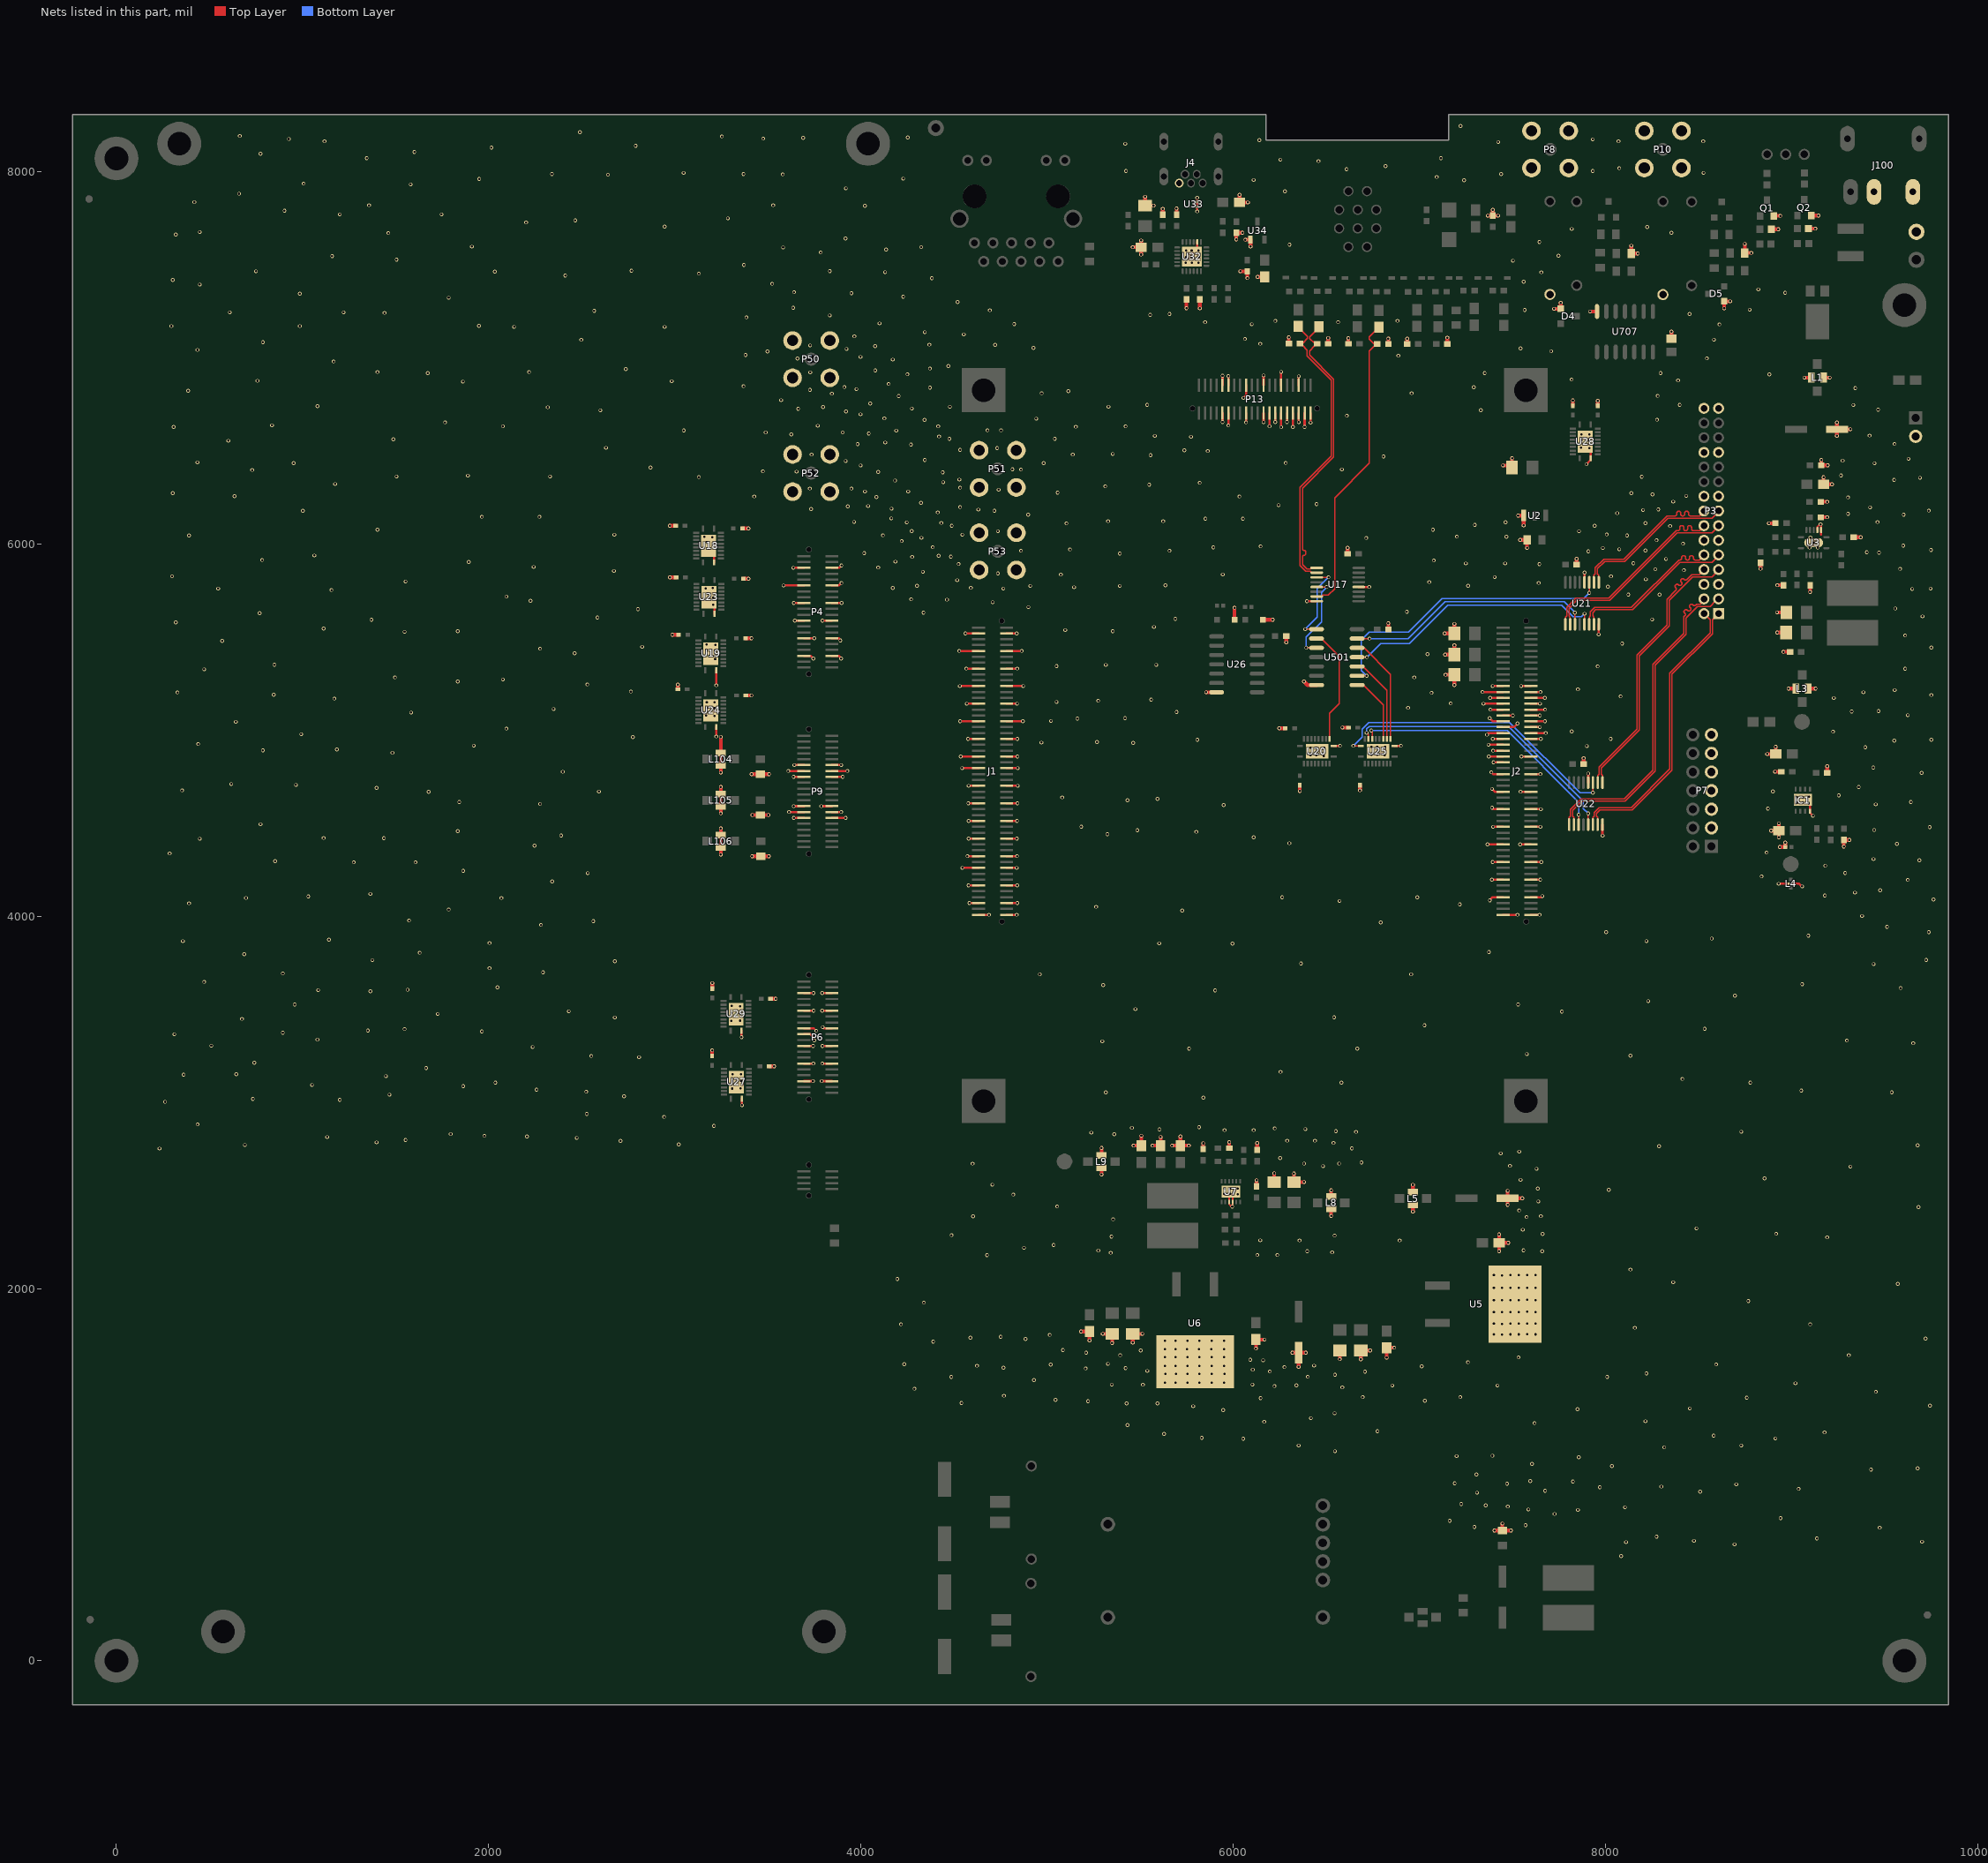
[diagram p0: the nets of this part, all layers, seen from the top]
# Altium PCB MISC82191.PcbDoc (part 6 of 9)
Units mil, origin at the board's own origin, x right, y up, seen from the top; angles counter-clockwise.
Board outline 10078.74 x 8543.31 mil, 4 copper layers (Top Layer, GND, POWER, Bottom Layer); 238 components, 299 nets, 1297 pads, 1665 vias.

## Via types
v1: diameter 20, hole 12, Top Layer to Bottom Layer, 1664 vias
v2: diameter 40, hole 20, Top Layer to Bottom Layer, 1 vias

## Nets (pads, with @x,y where several pads share a name; then routed paths per layer and width w, separated by ;. In a path a pad name is that pad's centre, name@x,y a point inside that pad or via, vN(x,y) a via of type N, cw(c..) or ccw(c..) an arc to the next point about the centre after c; other vN are vias at no path point) (continued)
DGND: (continued)
  other v1: 8084,563 8694,626 8110,638 9701,640 8475,645 9136,657 8275,667 9473,715 7296,719 7571,729 7163,752 8941,767 7726,789 7852,811 7586,813 8105,825 7475,829 7357,835 7225,842 7310,903 8509,909 7676,913 9038,924 7970,932 8300,936 8703,948 7471,951 7190,954 7825,963 7596,966 7307,1001 9427,1027 9677,1034 8035,1046 7605,1058 7857,1094 7200,1100 7393,1102 6547,1126 8316,1147 6352,1157 8730,1157 6054,1193 8913,1195 5831,1198 8581,1210 5629,1219 9177,1227 6775,1234 5432,1267 7619,1277 6167,1284 8215,1287 6417,1304 6544.78,1329.78 5946,1347 7850,1352 8453,1356 5785,1368 9744,1371 5427,1383 5593,1383 4540,1385 5220,1395 7030,1397 5045,1402 6146.78,1411.78 8759,1414 6696,1417 7220,1417 4768,1424 9453,1445 4288,1462 6586,1469 6221.78,1476.16 6855,1479 7420,1479 6339.78,1480.16 5514.78,1483.16 5347.78,1484.16 6103.78,1484.16 9021,1491 5633.78,1495.16 5690.78,1495.16 5753.78,1495.16 5817.78,1495.16 5883.78,1495.16 5951.78,1495.16 4929,1508 4485,1525 8009,1525 6400.78,1526.16 6547,1537 5634.78,1541.16 5691.78,1541.16 5754.78,1541.16 5818.78,1541.16 5884.78,1541.16 5952.78,1541.16 8220,1544 6196.78,1554.16 6708,1554 5538.78,1557.16 6104.78,1564.16 5207.78,1571.16 5421.78,1572.16 4766,1575 6274.78,1578.16 7013,1582 5633.78,1584.16 5690.78,1584.16 5753.78,1584.16 5817.78,1584.16 5883.78,1584.16 5951.78,1584.16 4624,1585 6434.78,1586.16 5019.78,1591.16 8595,1592 4232,1594 5326.78,1595.16 7261,1604 6160.78,1614.16 6091.78,1617.16 7533,1630 5633.78,1631.16 5690.78,1631.16 5753.78,1631.16 5817.78,1631.16 5883.78,1631.16 5951.78,1631.16 5392.78,1642.16 9307,1642 5209.78,1655.16 5502.78,1667.16 5084.78,1670.16 5632.78,1674.16 5689.78,1674.16 5752.78,1674.16 5816.78,1674.16 5882.78,1674.16 5950.78,1674.16 4388,1715 5633.78,1719.16 5690.78,1719.16 5753.78,1719.16 5817.78,1719.16 5883.78,1719.16 5951.78,1719.16 4884,1729 9720,1731 4588,1736 4751,1741 5013.78,1751.16 7445.4,1752.78 7400.4,1753.78 7488.4,1753.78 7535.4,1753.78 7624.4,1753.78 7578.4,1754.78 8158,1789 4215,1808 9100,1808 7445.4,1809.78 7400.4,1810.78 7488.4,1810.78 7535.4,1810.78 7624.4,1810.78 7578.4,1811.78 7445.4,1872.78 7400.4,1873.78 7488.4,1873.78 7535.4,1873.78 7624.4,1873.78 7578.4,1874.78 4338,1924 8768,1933 7445.4,1936.78 7400.4,1937.78 7488.4,1937.78 7535.4,1937.78 7624.4,1937.78 7578.4,1938.78 7445.4,2002.78 7400.4,2003.78 7488.4,2003.78 7535.4,2003.78 7624.4,2003.78 7578.4,2004.78 9571,2025 8364,2034 4195.53,2051 7445.4,2070.78 7400.4,2071.78 7488.4,2071.78 7535.4,2071.78 7624.4,2071.78 7578.4,2072.78 8134,2102 4677,2179 6129.78,2180.16 6236.78,2180.16 5341.78,2192.16 6531.78,2194.16 6397.78,2200.16 7659.78,2200.78 5275.78,2204.16 7559.4,2205.78 4876,2219 5035,2234 6356.78,2258.16 6894.78,2258.41 6145.78,2259.16 9191,2275 5345.78,2279.16 6544.78,2284.16 4487,2287 7662.78,2292.78 8917,2294 7555.4,2315.78 8489,2323 5354.78,2372.16 7576.4,2383.78 4602,2388 7652.78,2388.78 7535.78,2419.78 9682,2438 5054,2441 7639.78,2467.78 4819,2505 6023.78,2506.16 5951.78,2509.16 5984.78,2509.16 8018,2530 5984.78,2536.16 7636.78,2536.78 5952.78,2538.16 6023.78,2538.16 4706,2558 7543.78,2583.78 8855,2592 7629.78,2642.78 9316,2655 6482.78,2657.16 7487.4,2658.78 4600,2671 6380.78,2671.16 6568.78,2671.16 6688.78,2677.16 6251.78,2701.16 7437.4,2725.78 7536.4,2735.78 231,2752 6637.78,2753.16 8288,2765 9677,2770 690,2771 3021,2774 6538.78,2782.16 1397,2785 2708,2793 6289.78,2794.16 6439.78,2794.16 1553,2798 2473,2809 1132,2814 2206,2817 1977,2820 5360.78,2829.16 1796,2830 5237.78,2837.16 6659.78,2841.16 8730,2842 6551.78,2845.16 5953.78,2851.16 6109.78,2851.16 5603.78,2855.16 6387.78,2856.16 6222.78,2860.16 5455.78,2863.16 5816.78,2867.16 3210,2874 436,2882 2942,2922 2527,2938 261,3003 1199.78,3014.16 732.78,3018.16 5840,3025 2727,3033 1467,3041 5316,3054 9538,3054 2524,3057 9052,3063 2257,3068 3308.78,3074.16 3352.78,3075.16 1863,3087 1050.78,3093.16 2036,3106 6581,3106 8778,3106 3308.78,3115.16 3354.78,3115.16 8413,3126 1448,3141 361,3149 3309.78,3150.16 3354.78,3150.16 644,3151 6254,3164 1664,3184 740.78,3213.16 2808,3243 2551,3249 8134,3251 7577.78,3259.16 5763,3289 6667,3289 2236,3297 509.78,3304.16 9653,3318 5297,3328 9297,3332 1079.78,3337.16 310.78,3366.16 893.78,3374.16 1963,3381 1351,3386 1548,3394 8533,3395 7028,3414 3303.78,3438.16 3349.78,3439.16 674.78,3448.16 2678,3456 6542,3457 1726,3475 3349.78,3479.16 3305.78,3480.16 7765.78,3488.16 2430,3489 5475,3501 3349.78,3517.16 3304.78,3518.16 957.78,3525.16 7530.78,3526.16 8230,3544 8696,3573 1364,3597 5903,3602 1083.78,3603.16 1564,3605 9586,3614 2047,3618 5302,3630 9057,3635 471.78,3647.16 4961,3688 6956,3688 893.78,3692.16 2292,3699 2004,3721 9441,3743 6364,3746 2678,3758 1375,3764 9723,3765 686.78,3796.16 1629,3804 7374,3808 5995.78,3852.41 5602.78,3854.41 2004,3856 356.78,3866.16 8220,3866 1141.78,3874.16 8571,3880 9090,3895 8004,3914 9737,3914 9513,3943 2281,3953 6792,3967 2562,3974 1572,3977 9379,4001 5725.78,4030.16 1785,4036 5263.78,4050.16 7217.78,4064.16 389.78,4069.16 6571,4082 9763,4090 695.78,4098.16 2068,4098 6263,4102 6989,4102 1030.78,4106.16 9178.78,4111.16 1364,4120 9340.78,4127.16 9475.78,4139.16 2341,4187 9624,4195 8838.78,4214.16 2532,4231 9287.78,4232.16 1863,4244 9180.78,4271.16 1275,4290 1607,4290 852.78,4296.16 9687,4301 9439.78,4307.16 285.78,4337.16 8865.78,4342.16 2246,4379 9566,4388 6302,4392 447.78,4416.16 1437,4419 1112.78,4420.16 6110,4424 2389,4433 5324,4441 5802,4453 1834,4457 5485,4462 9443.78,4463.16 9742,4479 5184,4481 773.78,4494.16 8872.78,4578.16 5949,4597 9451.78,4601.16 2276,4603 9092.78,4607.16 9028.78,4610.16 9061.78,4611.16 1842,4614 9641,4614 5432,4623 5593,4630 5081,4638 9060.78,4638.16 9028.78,4639.16 9093.78,4641.16 9253.78,4649.16 1677,4668 2592,4670 8899.78,4670.16 352.78,4676.16 1397,4689 9360.78,4694.16 964.78,4705.16 616.78,4710.16 9699,4770 2398,4776 9439,4799 6487.78,4861.16 6414.78,4864.16 6446.78,4864.16 6814.78,4865.16 6741.78,4868.16 6773.78,4868.16 1483,4878 786.78,4891.16 1183.78,4896.16 6414.78,4906.16 6446.78,4906.16 6488.78,4906.16 9395.78,4907.16 6741.78,4910.16 6773.78,4910.16 6815.78,4910.16 7900,4914 1920,4916 438.78,4925.16 5463,4931 4970,4933 5268,4936 9552,4943 5807,4948 9751,4948 8028,4953 2775,4962 992.78,4978.16 9222.78,4991.16 7819,4993 2095,5008 641.78,5044.16 5021,5049 5162.78,5061.16 5418.78,5064.16 3213.78,5076.16 3168.78,5077.16 9624,5080 1583,5094 5696,5097 9322.78,5099.16 9466.78,5102.16 2349,5113 3171.78,5118.16 3213.78,5118.16 6939.78,5119.16 7168.78,5143.16 3171.78,5150.16 3213.78,5150.16 5050.78,5151.16 5274.78,5157.16 5558.78,5163.16 1170.78,5169.16 9226.78,5172.16 8081,5181 9751,5188 844.78,5189.16 7065.78,5200.16 327.78,5202.16 9386,5203 2764,5207 9554,5215 7852,5219 2530,5245 1834,5261 2076,5272 1496,5283 6972.78,5283.16 471.78,5326.16 9610,5330 7958,5342 5050.78,5344.16 5315.78,5350.16 5586.78,5350.16 848.78,5351.16 3216.78,5381.16 3186.78,5398.16 7043.78,5408.16 2462,5412 3216.78,5426.16 3170.78,5427.16 2276,5437 9751,5443 2824,5447 3217.78,5457.16 3169.78,5459.16 8090,5465 567.78,5479.16 9610,5508 1548,5528 1834,5531 5352.78,5531.16 5097.78,5537.16 1112.78,5545.16 5574,5554 318.78,5578.16 1370,5593 8251,5594 5689,5597 2584,5604 9703,5611 769.78,5628.16 4335.78,5630.41 6933,5635 2802,5650 9557,5653 4899.78,5660.41 3206.78,5674.16 4707.78,5686.41 2225,5695 4462.78,5700.41 4269.78,5702.41 3205.78,5710.16 2095,5717 8123,5728 8291,5728 3177.78,5732.16 1154.78,5752.16 9648,5758 546.78,5760.16 3165.78,5760.16 4764.78,5760.16 9747,5760 3203.78,5763.16 4170.78,5763.16 4590.78,5764.16 5144.78,5767.16 8013,5770 4909.78,5774.16 5390.78,5774.16 4300.78,5775.41 7262,5775 5635.78,5777.16 7641,5790 7053,5795 1553,5798 4516.78,5805.16 8217,5810 7405,5822 298.78,5826.16 8030,5826 5073.78,5835.41 5943.78,5836.16 4735.78,5841.16 4332.78,5850.16 2673,5855 8422,5859 8268,5864 9583,5866 4092.78,5873.16 2241,5876 7645,5891 4524.78,5892.16 7250,5895 7461,5895 8150,5896 1893,5903 4184.78,5904.41 7078,5911 782.78,5913.16 8325,5919 4274.78,5930.16 4482.78,5931.41 4417.78,5936.16 1063.78,5938.16 5390.78,5948.16 4017.78,5950.78 9469.78,5953.16 9403.78,5955.16 7908,5960 4859.78,5963.16 5657.78,5963.16 8215,5965 9749,5967 5122.78,5970.16 8074,5971 3182.78,5975.16 7986,5978 9096.78,5980.16 9140.78,5980.16 5893,5981 4385.78,5982.41 6146.78,5987.16 9600,5991 3206.78,6000.16 8417,6001 9116.78,6007.16 3171.78,6010.16 4218.78,6015.16 8275,6020 4324.78,6032.41 6714.78,6032.16 9100.78,6034.16 3201.78,6035.16 3157.78,6038.16 7468,6038 7202,6039 389.78,6045.16 8116,6045 4117.78,6046.41 2675,6049 4544.78,6049.41 8007,6051 4735.78,6068.16 7858,6068 4272.78,6069.16 1402,6076 7073,6076 8347.78,6096 4487.78,6097.16 7942,6097 7298,6102 5103.78,6110.16 4431.78,6112.41 8215,6112 4245.78,6115.41 7463,6116 9461.78,6117.16 3962.78,6117.78 5327.78,6122.16 5623.78,6122.16 5850.78,6135.16 6052,6135 4162.78,6137.16 1963,6146 2273,6146 4898.78,6157.16 9602,6157 9303.78,6161.16 8063,6165 4412.78,6169.16 1001.78,6178.16 4716.78,6178.16 9737,6179 8202,6182 4630.78,6184.16 8284,6185 3732.78,6188 4164.78,6189.41 9421.78,6196.16 4532.78,6198.16 3928.78,6201.78 4037.78,6203.41 6243.78,6208.16 6447.78,6214.16 4322.78,6220.41 8364,6227 9303.78,6250.16 4082.78,6251.41 3427,6255 6033,6255 633.78,6256.16 8434,6258 8253,6266 302.78,6273.16 8139,6273 5056.78,6275.16 4021.78,6281.41 4253.78,6281.41 4739.78,6291.16 3724.78,6297.41 3948.78,6297.41 4532.78,6302.16 5312.78,6309.16 5548.78,6318.16 1174.78,6322.16 5819.78,6328.16 4441.78,6331.16 4183.78,6340.41 9551,6344 4528.78,6345.41 9690,6355 3129,6359 8195,6361 1505,6362 2330,6362 1888,6367 9265.78,6368.16 4439.78,6384.41 4092.78,6386.41 3653.78,6388.41 3473,6390 728.78,6397.16 4859.78,6399.16 6583.78,6400.16 4813.78,6401.41 2870,6410 3998.78,6421.41 9446,6433 951.78,6434.16 4981.78,6434.41 6281.78,6435.16 434.78,6438.16 3917.78,6445.41 9273.78,6447.16 4342.78,6450.41 9628,6457 6807.78,6470.16 5555.78,6477.16 3734.78,6480.16 5137.78,6480.16 5352.78,6483.16 5863.78,6499.16 5737.78,6502.41 4532.78,6505.16 4731.78,6515.16 7913.78,6515.16 2630,6516 7868.78,6516.16 4268.78,6533.41 3981.78,6535.78 9553,6537 4130.78,6544.41 600.78,6554.16 7871.78,6557.16 7913.78,6557.16 1488,6562 5041.78,6564.41 4474.78,6564.78 5772.78,6575.41 4419.78,6577.41 5578.78,6580.41 9419,6582 3625.78,6588.16 7871.78,6589.16 7913.78,6589.16 4041.78,6593.41 3487.78,6598.78 3901.78,6598.78 4189.78,6608.41 3048,6610 4679.78,6610.41 4752.78,6610.41 306.78,6628.16 5154.78,6629.41 5421.78,6631.41 2076,6632 4414.78,6631.78 3767.78,6634.78 835.78,6637.16 1766,6653 4341.78,6666.41 8277,6667 4941.78,6672.41 4125.78,6674.41 6610.78,6688.41 3997.78,6696.41 3919.78,6711.78 2600,6718 7330.78,6718.16 9465,6721 3662.78,6725.78 4273.78,6727.41 2317,6734 3796.78,6735.41 4477.78,6736.41 5329.78,6736.41 1079.78,6740.16 9332,6746 5537.78,6747.41 8399,6747 4049.78,6754.41 3570.78,6772.41 4202.78,6794.41 8280,6795 3843.78,6807.16 4970.78,6809.41 6958.78,6809.16 5113.78,6820.41 385.78,6823.16 3725.78,6827.78 3975.78,6831.41 9342,6837 4370.78,6839.16 3910.78,6842.4 7292.78,6842.16 3368.78,6847.41 4148.78,6859.41 1861,6872 2983,6874 757.78,6876.16 8390,6878 7817.78,6883.16 8880.78,6910.16 4249.78,6911.16 1672,6918 7351,6918 8296,6918 3727.78,6921.41 1402,6923 2217,6923 4076.78,6931.41 2737,6939 4370.78,6942.16 4469.78,6955.41 1166.78,6980.16 4170.78,6990.16 3658.78,6995.41 8545,6996.81 3997.78,7004.41 6887.78,7011.16 3379.78,7014.41 3497.78,7033.41 7708,7035 434.78,7042.16 3922.78,7047.41 7544,7050 4926.78,7053.16 4075.78,7062.16 3726.78,7066.41 4720.78,7069.16 4367.78,7070.16 6145.78,7075.16 786.78,7083.16 2497,7096 8583,7097 6063,7101 3964.78,7115.16 4552.78,7125.16 4342.78,7137.16 2136,7166 2945,7166 294.78,7170.16 984.78,7170.16 1947,7171 8612,7179 6099.78,7180.16 4823.78,7181.16 4099.78,7184.41 5849,7191 6563.78,7191.16 6227,7198 6882.78,7198.16 3384.78,7217.41 3832.78,7227.41 5554,7231 5658,7235 8452,7235 1440,7241 608.78,7244.16 1220.78,7244.16 2567,7252 4692.78,7255.16 7566,7257 8775,7258 3635.78,7268.41 4518.78,7299.16 1785,7322 4226.78,7327.41 984.78,7344.16 3948.78,7346.41 8965,7349 3640.78,7352.41 8821,7367 447.78,7393.16 3522.78,7397.41 7560,7408 302.78,7418.16 4380.78,7427.41 2411,7441 3129,7452 4129.78,7459.41 7654.78,7459.16 2033,7463 749.78,7464.16 3832.78,7465.41 2767,7468 3371,7498 5744.78,7509.16 5813.78,7509.16 5778.78,7510.16 7503,7521 1505,7527 5814.78,7541.16 5747.78,7542.16 5777.78,7542.16 1158.78,7546.16 7747.78,7548.16 3783.78,7565.41 5812.78,7576.16 5746.78,7577.16 5776.78,7577.16 4134.78,7581.41 3581.78,7592.41 4323.78,7594.41 1909,7597 6302.78,7607.16 7644.78,7621.16 3916.78,7640.41 318.78,7662.16 1460.78,7670.16 8354.78,7671.16 447.78,7675.16 7818.78,7692.16 8223.78,7702.16 2945,7705 2201,7727 2465,7738 3285,7749 1199.78,7770.16 1747,7770 902.78,7790.16 4022,7816 1356.78,7819.16 3528,7819 418.78,7836.16 658.78,7881.16 6277.78,7894.16 3919,7910 1580.78,7931.16 1005.78,7935.16 7240,7954 6109.78,7955.16 1948.78,7960.16 4227,7962 7094,7971 2640.78,7983.16 3579.78,7985.16 2339.78,7987.16 3368.78,7987.16 7439.78,7987.16 3046.78,7993.16 8526.78,7993.16 5423.78,8003.16 7931.78,8003.16 6609,8013 8073.78,8018.16 6819,8029 6458,8056 6253.78,8064.16 1344.78,8072.16 7116,8072 773.78,8096.16 1600.78,8105.16 2014.78,8129.16 2789.78,8138.16 5419.78,8149.16 7423.78,8159.16 1117.78,8163.16 8069.78,8163.16 8524.78,8163.16 6140.78,8169.16 7931.78,8173.16 926.78,8175.16 3474.78,8177.16 3689.78,8181.16 4251,8183 3252.78,8189.16 662.78,8191.16 2489.78,8212.16 7221,8245
"ENCODER2 A": U21.3 U501.13 | length 1302.2
  Top Layer w6: U501.13@6665.7,5491.72 v1(6732.21,5491.72) ; U21.3@7835.78,5599.16 v1(7835.78,5630.16)
  Bottom Layer w6: v1(6732.21,5491.72) 6940.35,5491.72 7137.78,5689.16 7778.78,5689.16 v1@7832.78,5635.16
"ENCODER2 A+": P3.13 U21.2 | length 1075
  Top Layer w6: U21.2@7810.37,5568.16 7810.37,5606.16 7803.57,5612.95 7803.57,5654.2 7845.78,5696.41 8023.41,5696.41 8386.41,6059.41 8573.78,6059.41 P3.13@8607.78,6093.41
"ENCODER2 A-": P3.14 U21.1 | length 1074
  Top Layer w6: U21.1@7784.78,5568.16 7784.78,5606.16 7791.57,5612.95 7791.57,5659.17 7840.81,5708.41 8018.44,5708.41 8381.44,6071.41 8389,6071.41 8390.05,6071.41 ccw(c8390.05,6080.86) 8399.5,6080.86 8399.5,6089.03 cw(c8408.95,6089.03) 8408.95,6098.48 8411.05,6098.48 cw(c8411.05,6089.03) 8420.5,6089.03 8420.5,6080.86 ccw(c8429.95,6080.86) 8429.95,6071.41 8432.05,6071.41 ccw(c8432.05,6080.86) 8441.5,6080.86 8441.5,6089.03 cw(c8450.95,6089.03) 8450.95,6098.48 8453.05,6098.48 cw(c8453.05,6089.03) 8462.5,6089.03 8462.5,6080.86 ccw(c8471.95,6080.86) 8471.95,6071.41 8483,6071.41 8506.78,6071.41 P3.14@8519.78,6084.41
"ENCODER2 AA": U25.12 U501.12 | length 567.6
  Top Layer w6: U501.12@6682.78,5441.16 6703.78,5441.16 6845.25,5299.68 U25.12@6845.25,4953.18
"ENCODER2 B": U21.5 U501.11 | length 1399.3
  Top Layer w6: U501.11@6665.7,5391.72 v1(6718.35,5391.72) ; U21.5@7887.78,5595.16 v1(7887.78,5625.16)
  Bottom Layer w6: v1(6718.35,5391.72) 6791.78,5465.16 6946.78,5465.16 7151.78,5670.16 7764.78,5670.16 7825.78,5609.16 7871.78,5609.16 v1(7887.78,5625.16)
"ENCODER2 B+": P3.10 U21.6 | length 866
  Top Layer w6: U21.6@7912.74,5568.16 7912.74,5606.16 7919.53,5612.95 7919.53,5636.38 7942.56,5659.41 8139.81,5659.41 8393.81,5913.41 8399,5913.41 8400.05,5913.41 ccw(c8400.05,5922.86) 8409.5,5922.86 8409.5,5927.33 cw(c8418.95,5927.33) 8418.95,5936.78 8421.05,5936.78 cw(c8421.05,5927.33) 8430.5,5927.33 8430.5,5922.86 ccw(c8439.95,5922.86) 8439.95,5913.41 8442.05,5913.41 ccw(c8442.05,5922.86) 8451.5,5922.86 8451.5,5927.33 cw(c8460.95,5927.33) 8460.95,5936.78 8463.05,5936.78 cw(c8463.05,5927.33) 8472.5,5927.33 8472.5,5922.86 ccw(c8481.95,5922.86) 8481.95,5913.41 8487,5913.41 8504.78,5913.41 P3.10@8528.78,5937.41
"ENCODER2 B-": P3.9 U21.7 | length 866.2
  Top Layer w6: U21.7@7938.33,5568.16 7938.33,5606.16 7931.53,5612.95 7931.53,5631.41 7947.53,5647.41 8144.78,5647.41 8398.78,5901.41 8571.78,5901.41 P3.9@8605.78,5935.41
"ENCODER2 BB": U25.13 U501.10 | length 442.3
  Top Layer w6: U501.10@6696.78,5342.16 6825.57,5213.37 U25.13@6825.57,4953.18
"ENCODER2 Z": U21.11 U501.9 | length 1612.4
  Top Layer w6: U501.9@6665.7,5291.72 v1(6717.21,5291.72) ; v1(7912.78,5737.16) U21.11@7912.78,5764.16
  Bottom Layer w6: v1(6717.21,5291.72) 6687.78,5321.16 6687.78,5483.16 6729.78,5525.16 6940.78,5525.16 7122.78,5707.16 7882.78,5707.16 v1(7912.78,5737.16)
"ENCODER2 Z+": P3.16 U21.10 | length 843
  Top Layer w6: U21.10@7938.33,5793.81 7938.33,5831.16 7945.12,5837.95 7945.12,5872.38 7991.15,5918.41 8099.44,5918.41 8331.44,6150.41 8373,6150.41 8374.05,6150.41 ccw(c8374.05,6159.86) 8383.5,6159.86 8383.5,6165.57 cw(c8392.95,6165.57) 8392.95,6175.02 8395.05,6175.02 cw(c8395.05,6165.57) 8404.5,6165.57 8404.5,6159.86 ccw(c8413.95,6159.86) 8413.95,6150.41 8416.05,6150.41 ccw(c8416.05,6159.86) 8425.5,6159.86 8425.5,6165.57 cw(c8434.95,6165.57) 8434.95,6175.02 8437.05,6175.02 cw(c8437.05,6165.57) 8446.5,6165.57 8446.5,6159.86 ccw(c8455.95,6159.86) 8455.95,6150.41 8479,6150.41 8505.78,6150.41 P3.16@8519.78,6164.41
"ENCODER2 Z-": P3.15 U21.9 | length 843.9
  Top Layer w6: U21.9@7963.92,5793.81 7963.92,5831.16 7957.12,5837.95 7957.12,5867.41 7996.12,5906.41 8104.41,5906.41 8336.41,6138.41 8572.78,6138.41 P3.15@8600.78,6166.41
"ENCODER2 ZZ": U25.14 U501.8 | length 331.5
  Top Layer w6: U501.8@6700.78,5241.16 6805.88,5136.06 U25.14@6805.88,4953.18
"ENCODER3 A": U22.3 U25.17 | length 1439.4
  Top Layer w6: v1(6741.78,4997.16) 6746.83,4992.11 U25.17@6746.83,4953.18 ; U22.3@7855.96,4492.16 v1(7855.96,4544.98)
  Bottom Layer w6: v1(6741.78,4997.16) 7471.78,4997.16 7856.78,4612.16 v1@7856.78,4549.16 ; v1@7854.78,4546.16 v1@7854.78,4549.16
"ENCODER3 A+": P3.3 U22.2 | length 1695.3
  Top Layer w6: U22.2@7830.37,4492.16 7830.37,4530.16 7823.57,4536.95 7823.57,4568.41 7873.57,4618.41 8105.75,4618.41 8267.78,4780.44 8267.78,5347.41 8433.78,5513.41 8433.78,5602.81 8434,5603.03 8434,5603.63 ; 8434,5603.66 8494.75,5664.41 8562.78,5664.41 P3.3@8589.78,5691.41
"ENCODER3 A-": P3.4 U22.1 | length 1695
  Top Layer w6: U22.1@7804.78,4492.16 7804.78,4530.16 7811.57,4536.95 7811.57,4573.38 7868.6,4630.41 8100.78,4630.41 8255.78,4785.41 8255.78,5352.38 8421.78,5518.38 8421.78,5608.38 8422,5608.6 8426.19,5612.81 8426.93,5613.56 ccw(c8420.25,5620.24) 8426.93,5626.92 8424.58,5629.27 cw(c8431.26,5635.95) 8424.58,5642.64 8426.06,5644.12 cw(c8432.74,5637.44) 8439.43,5644.12 8441.78,5641.77 ccw(c8448.46,5648.45) 8455.14,5641.77 8456.63,5643.26 ccw(c8449.94,5649.94) 8456.63,5656.62 8454.28,5658.97 cw(c8460.96,5665.65) 8454.28,5672.34 8455.76,5673.82 cw(c8462.44,5667.14) 8469.12,5673.82 8471.48,5671.47 ccw(c8478.16,5678.15) 8484.84,5671.47 8487.19,5673.81 8489.78,5676.41 8508.78,5676.41 P3.4@8519.78,5687.41
"ENCODER3 B": U22.5 U25.18 | length 1530.6
  Top Layer w6: v1(6716.99,4985.18) 6718.76,4985.18 6727.14,4976.8 U25.18@6727.14,4953.18 ; U22.5@7907.15,4492.16 v1(7907.15,4551.53)
  Bottom Layer w6: v1(6716.99,4985.18) 6716.99,5006.36 6729.78,5019.16 7478.78,5019.16 7879.78,4618.16 7879.78,4579.16 v1@7907.78,4551.16
"ENCODER3 B+": P3.2 U22.6 | length 1508.8
  Top Layer w6: U22.6@7932.74,4492.16 7932.74,4530.16 7939.53,4536.95 7939.53,4556.38 7966.56,4583.41 8138.78,4583.41 8345.78,4790.41 8345.78,5305.38 8562,5521.6 8562,5592.82 P3.2@8529.04,5625.78
"ENCODER3 B-": P3.1 U22.7 | length 1509.5
  Top Layer w6: U22.7@7958.33,4492.16 7958.33,4530.16 7951.53,4536.95 7951.53,4551.41 7971.53,4571.41 8143.75,4571.41 8357.78,4785.44 8357.78,5300.41 8574,5516.63 8574,5592.63 8607.15,5625.78 P3.1@8607.78,5625.78
"ENCODER3 Z": U22.11 U25.20 | length 1596.9
  Top Layer w6: v1(6645.4,4915.78) U25.20@6685.8,4915.78 ; v1(7932.78,4663.16) 7932.78,4697.16 U22.11@7933.78,4698.16
  Bottom Layer w6: v1(6645.4,4915.78) 6691.78,4962.16 6691.78,5005.16 6727.78,5041.16 7485.78,5041.16 7863.78,4663.16 v1(7932.78,4663.16)
"ENCODER3 Z+": P3.8 U22.10 | length 1453
  Top Layer w6: U22.10@7958.33,4717.81 7958.33,4755.16 7965.12,4761.95 7965.12,4800.38 8168.78,5004.03 8168.78,5402.38 8329.78,5563.38 8329.78,5702.38 8377.7,5750.3 8378.44,5751.04 ccw(c8371.76,5757.72) 8378.44,5764.41 8376.71,5766.14 cw(c8383.39,5772.82) 8376.71,5779.5 8378.2,5780.99 cw(c8384.88,5774.3) 8391.56,5780.99 8393.29,5779.26 ccw(c8399.97,5785.94) 8406.66,5779.26 8408.14,5780.74 ccw(c8401.46,5787.42) 8408.14,5794.11 8406.41,5795.84 cw(c8413.09,5802.52) 8406.41,5809.2 8407.9,5810.68 cw(c8414.58,5804) 8421.26,5810.68 8422.99,5808.95 ccw(c8429.67,5815.64) 8436.35,5808.95 8462.81,5835.41 8503.78,5835.41 P3.8@8526.78,5858.41
"ENCODER3 Z-": P3.7 U22.9 | length 1453.8
  Top Layer w6: U22.9@7983.92,4717.81 7983.92,4755.16 7977.12,4761.95 7977.12,4795.41 8180.78,4999.06 8180.78,5397.41 8341.78,5558.41 8341.78,5697.41 8467.78,5823.41 8571.78,5823.41 P3.7@8598.78,5850.41
"ENCODER A": U17.3 U501.1 | length 447.2
  Top Layer w6: v1(6387.21,5541.72) U501.1@6447.66,5541.72 ; U17.3@6448.78,5819.98 v1@6505.96,5819.98
  Bottom Layer w6: v1(6387.21,5541.72) 6451.78,5606.29 6451.78,5761.16 v1@6510.78,5820.16
  other v1: 6511.78,5821.16
"ENCODER A_N": C55.1 L14.1 U17.1 | length 1572
  Top Layer w6: C55.1@6439.78,7072.16 C55.1@6436.78,7075.16 ; U17.1@6448.78,5871.16 6420.78,5871.16 6413.98,5864.36 6395.55,5864.36 6371.78,5888.13 6371.78,5900.16 6371.78,5913.16 6371.78,5930.06 cw(c6380.88,5930.06) 6380.88,5939.16 ccw(c6380.88,5948.26) 6389.98,5948.26 6389.98,5956.06 ccw(c6380.88,5956.06) 6380.88,5965.16 cw(c6380.88,5974.26) 6371.78,5974.26 6371.78,6003.16 6371.78,6299.16 6539.78,6467.16 6539.78,6884.13 6409.78,7014.13 6409.78,7037.16 6436.78,7064.16 C55.1@6436.78,7075.16 ; C55.1@6450.78,7075.16 C55.1@6436.78,7075.16 ; L14.1@6460.78,7166.16 6460.78,7161.16 6411.78,7112.16 6411.78,7103.16 6436.78,7078.16 C55.1@6436.78,7075.16
"ENCODER A_P": C54.1 L13.1 U17.2 | length 1571.9
  Top Layer w6: L13.1@6349.78,7168.16 6349.78,7165.16 6399.78,7115.16 6399.78,7104.16 C54.1@6371.78,7076.16 ; C54.1@6358.78,7076.16 C54.1@6371.78,7076.16 ; C54.1@6369.78,7074.16 C54.1@6371.78,7076.16 ; U17.2@6448.78,5845.57 6419.37,5845.57 6412.57,5852.36 6390.57,5852.36 6359.78,5883.16 6359.78,6304.13 6527.78,6472.13 6527.78,6879.16 6397.78,7009.16 6397.78,7040.16 6371.78,7066.16 C54.1@6371.78,7076.16
"ENCODER AA": U20.12 U501.2 | length 590.6
  Top Layer w6: U501.2@6479.78,5485.16 6569.78,5395.16 6569.78,5141.16 6518.25,5089.63 U20.12@6518.25,4953.18
"ENCODER B": U17.5 U501.3 | length 448.1
  Top Layer w6: v1(6392.78,5442.16) U501.3@6416.78,5442.16 ; U17.5@6448.78,5768.79 v1(6502.15,5768.79)
  Bottom Layer w6: v1(6392.78,5442.16) v1@6394.78,5444.16 ; v1@6392.78,5446.16 6392.78,5500.16 6473.78,5581.16 6473.78,5740.42 v1(6502.15,5768.79)
"ENCODER B_N": C60.1 L16.1 U17.7 | length 1654.4
  Top Layer w6: U17.7@6448.78,5717.61 6475.23,5717.61 6482.02,5724.4 6510.02,5724.4 6544.78,5759.16 6544.78,6247.16 6731.78,6434.16 6731.78,7036.16 6769.78,7074.16 C60.1@6773.78,7074.16 ; C60.1@6761.78,7069.16 6731.78,7099.16 6731.78,7112.16 L16.1@6783.78,7164.16